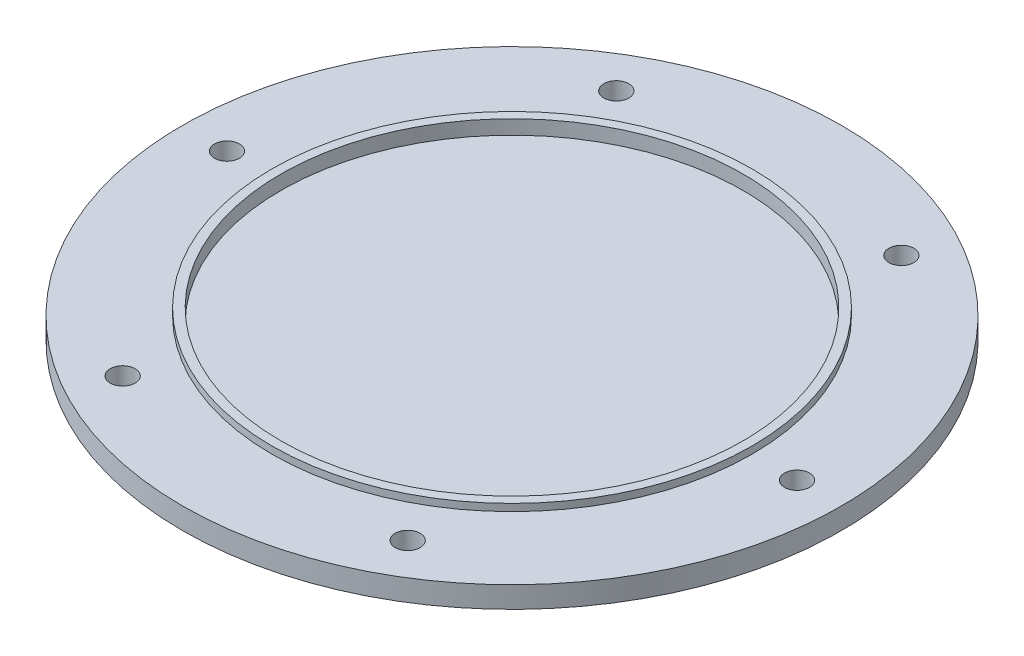
SolidWorks part; units mm, degrees
material "Gray Cast Iron"
ref_plane "Front Plane" through (0, 0, 0) normal (0, 0, 1) x (1, 0, 0)
ref_plane "Top Plane" through (0, 0, 0) normal (0, 1, 0) x (1, 0, 0)
ref_plane "Right Plane" through (0, 0, 0) normal (1, 0, 0) x (0, 0, -1)
sketch "Sketch1" plane through (0, 0, 0) normal (0, 1, 0) x (1, 0, 0)
  circle A0 centre (0, 0) radius 185
  dimension "D1" = 370
extrude "Boss-Extrude1" add sketch "Sketch1" along normal blind 12
sketch "Sketch2" plane through (0, 12, 0) normal (0, 1, 0) x (1, 0, 0)
  circle A0 centre (0, 0) radius 129.75
  dimension "D1" = 259.5
extrude "Cut-Extrude1" cut sketch "Sketch2" against normal blind 4
sketch "Sketch3" plane through (0, 12, 0) normal (0, 1, 0) x (1, 0, 0)
  circle A0 centre (0, 0) radius 129.75 construction
  circle A1 centre (0, 0) radius 129.75
  circle A2 centre (0, 0) radius 134.75
  dimension "D1" = 269.5
extrude "Boss-Extrude2" add sketch "Sketch3" along normal blind 4
sketch "Sketch5" plane through (0, 12, 0) normal (0, 1, 0) x (1, 0, 0)
  line L0 (0, 0) -> (160, 0) construction
  circle A0 centre (0, 0) radius 160 construction
  circle A1 centre (160, 0) radius 7
  dimension "D1" = 320
  dimension "D2" = 14
extrude "Cut-Extrude3" cut sketch "Sketch5" against normal through all
pattern_circular "CirPattern2" count 6 over 360 about axis through (0, 0, 0) along (0, 1, 0) of "Cut-Extrude3"
